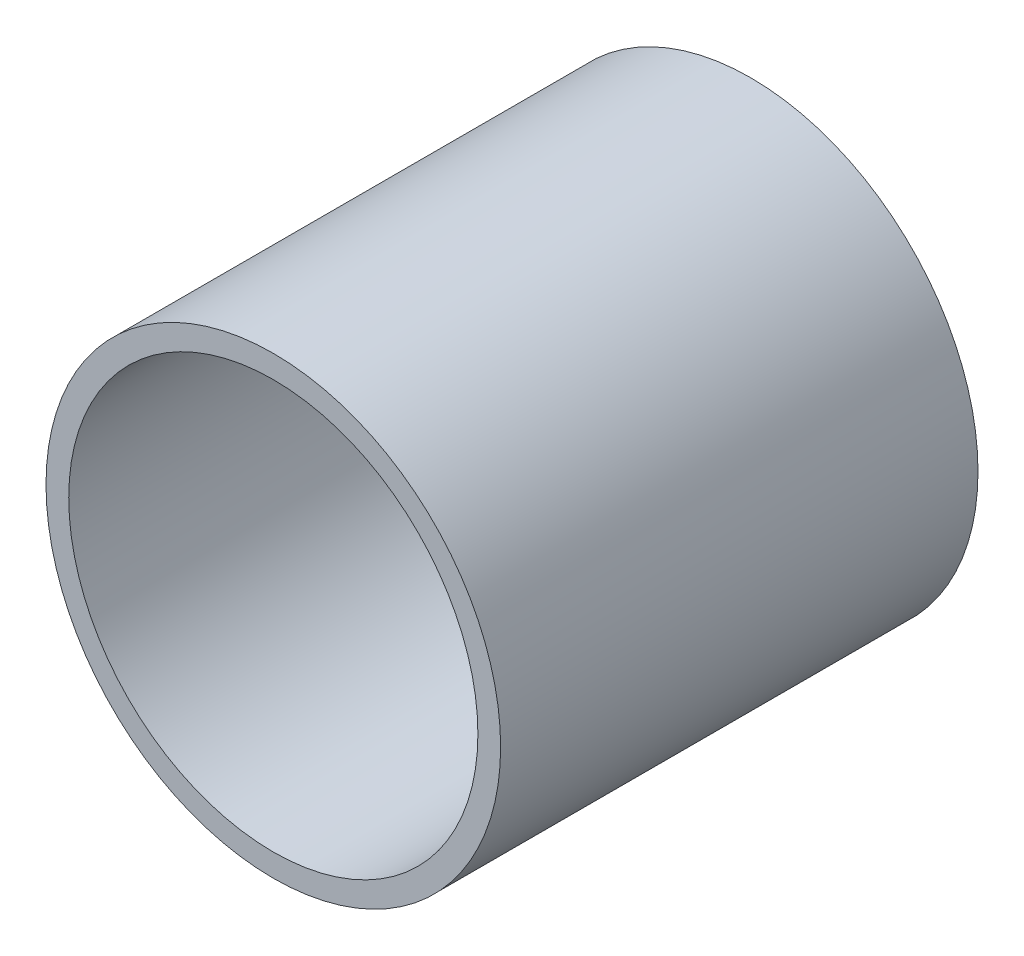
from build123d import *

# Parameters (mm, degrees)
SKETCH_1_R      = 10
SKETCH_1_R_2    = 9
EXTRUDE_1_DEPTH = 21


with BuildPart() as part:
    # 草图1 → 凸台-拉伸1 (new body)
    with BuildSketch(Plane.XY):
        with Locations(Location((0, 0, 0), (0, 0, 180))):
            Circle(SKETCH_1_R)
        with Locations(Location((0, 0, 0), (0, 0, 180))):
            Circle(SKETCH_1_R_2, mode=Mode.SUBTRACT)
    extrude(amount=EXTRUDE_1_DEPTH)


solid = part.part
